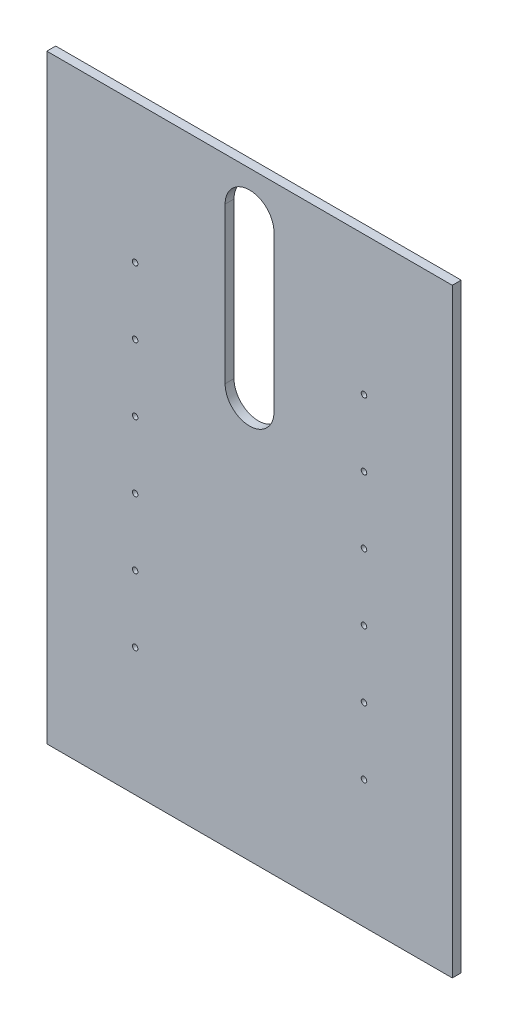
SolidWorks part; units mm, degrees
material "普通碳钢"
ref_plane "Front Plane" through (0, 0, 0) normal (0, 0, 1) x (1, 0, 0)
ref_plane "Top Plane" through (0, 0, 0) normal (0, 1, 0) x (1, 0, 0)
ref_plane "Right Plane" through (0, 0, 0) normal (1, 0, 0) x (0, 0, -1)
sketch "Sketch1" plane through (0, 0, 0) normal (0, 0, 1) x (1, 0, 0)
  line L1 (0, 0) -> (365, 0)
  line L2 (0, 0) -> (0, -540)
  line L3 (0, -540) -> (365, -540)
  line L4 (365, 0) -> (365, -540)
  line L8 (182.5, 0) -> (182.5, -540) construction
  line L9 (182.5, -39) -> (182.5, -179) construction
  line L10 (204.5, -39) -> (204.5, -179)
  line L11 (160.5, -39) -> (160.5, -179)
  arc A0 (204.5, -39) -> (160.5, -39) centre (182.5, -39) ccw
  arc A1 (160.5, -179) -> (204.5, -179) centre (182.5, -179) ccw
  point P16 (182.5, -109)
  dimension "D1" = 39
  dimension "D2" = 44
  dimension "D3" = 140
  dimension "D4" = 365
  dimension "D5" = 540
extrude "Boss-Extrude1" add sketch "Sketch1" along normal blind 8 contours L1 L4 L3 L2
hole_wizard "M6 Tapped Hole1" positions "Sketch2" profile "Sketch3" tap size "M6" standard "GB" end condition through all
sketch "Sketch2" plane through (0, 0, 8) normal (0, 0, 1) x (1, 0, 0)
  line L0 (182.5, -17) -> (182.5, -201) construction
  line L2 (365, 0) -> (0, 0) construction
  arc A0 (204.5, -39) -> (160.5, -39) centre (182.5, -39) ccw construction
  arc A1 (160.5, -179) -> (204.5, -179) centre (182.5, -179) ccw construction
  point P0 (79.5, -125)
  point P2 (285.5, -125)
  dimension "D1" = 206
  dimension "D2" = 125
sketch "Sketch3" plane through (79.5, -125, 8) normal (1, 0, 0) x (0, -1, 0)
  line L0 (0, 0) -> (0, 8)
  line L1 (0, 8) -> (2.5, 8)
  line L2 (2.5, 8) -> (2.5, 0)
  line L5 (2.5, 0) -> (0, 0)
  line L11 (0, -6.35) -> (0, 107.95) construction
  dimension "通孔螺纹孔钻头直径" = 5
  dimension "通孔螺纹孔钻头深度" = 8
cosmetic thread "Cosmetic Thread1" parameters "D2"=6
cosmetic thread "Cosmetic Thread2" parameters "D2"=6
pattern_linear "LPattern1" count 6 spacing 60 along (0, -1, 0) of "M6 Tapped Hole1"
